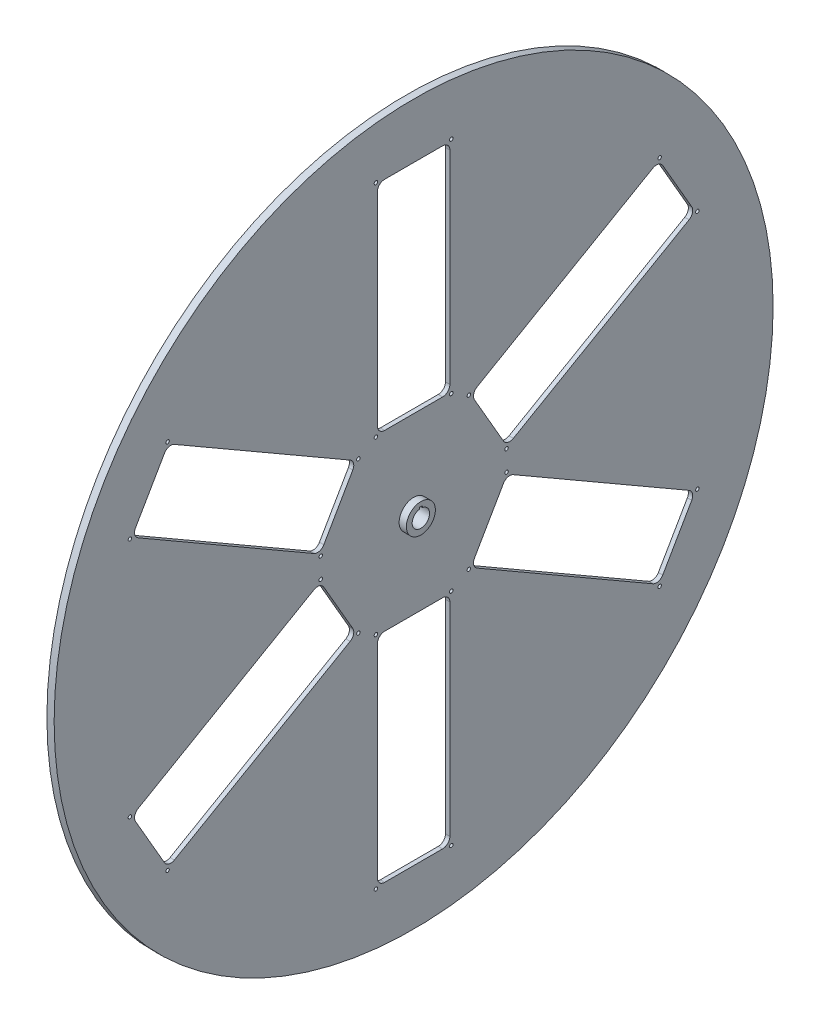
SolidWorks part; units mm, degrees
material "AISI 304"
ref_plane "Front Plane" through (0, 0, 0) normal (0, 0, 1) x (1, 0, 0)
ref_plane "Top Plane" through (0, 0, 0) normal (0, 1, 0) x (1, 0, 0)
ref_plane "Right Plane" through (0, 0, 0) normal (1, 0, 0) x (0, 0, -1)
sketch "Sketch1" plane through (0, 0, 0) normal (1, 0, 0) x (0, 0, -1)
  circle A0 centre (0, 0) radius 250
  dimension "D1" = 500
extrude "Boss-Extrude1" add sketch "Sketch1" along normal blind 5
sketch "Sketch5" plane through (0, 0, 0) normal (-1, 0, 0) x (0, 0, 1)
  line L0 (0, 0) -> (0, 425.8761) construction
  line L2 (-25, 210) -> (25, 210)
  line L3 (-25, 210) -> (-25, 60)
  line L4 (-25, 60) -> (25, 60)
  line L5 (25, 210) -> (25, 60)
  line L6 (-25, 210) -> (25, 60) construction
  line L7 (-25, 60) -> (25, 210) construction
  point P3 (0, 135)
  dimension "D1" = 50
  dimension "D2" = 60
  dimension "D3" = 150
extrude "Cut-Extrude1" cut sketch "Sketch5" against normal through all
pattern_circular "CirPattern1" count 6 over 360 about axis through (0, 0, 0) along (1, 0, 0) of "Cut-Extrude1"
sketch "Sketch6" plane through (0, 0, 0) normal (-1, 0, 0) x (0, 0, 1)
  line L8 (-30, 55) -> (30, 55)
  line L9 (30, 55) -> (30, 215)
  line L10 (-30, 215) -> (-30, 55)
  line L11 (30, 215) -> (-30, 215)
  line L12 (-30, 55) -> (30, 55)
  line L13 (30, 55) -> (30, 215)
  line L14 (-30, 215) -> (-30, 55)
  line L15 (30, 215) -> (-30, 215)
  dimension "D1" = 5
extrude "Cut-Extrude2" cut sketch "Sketch6" against normal blind 2
sketch "Sketch7" plane through (2, 0, 0) normal (-1, 0, 0) x (0, 0, 1)
  circle A0 centre (-26, 211) radius 1
  circle A1 centre (26, 211) radius 1
  circle A2 centre (-26, 59) radius 1
  circle A3 centre (26, 59) radius 1
extrude "Cut-Extrude3" cut sketch "Sketch7" against normal blind 10
hole_wizard "M2 Clearance Hole1" positions "Sketch8" profile "Sketch9" hole size "M2" standard "GB"
sketch "Sketch8" plane through (2, 0, 0) normal (-1, 0, 0) x (0, 0, 1)
  point P0 (-26, 59)
  point P3 (-26, 211)
  point P6 (26, 211)
  point P9 (26, 59)
sketch "Sketch9" plane through (2, 59, -26) normal (0, 1, 0) x (0, 0, 1)
  line L0 (0, 0) -> (0, 8.221)
  line L1 (0, 8.221) -> (1.2, 7.5)
  line L2 (1.2, 7.5) -> (1.2, 0)
  line L5 (1.2, 0) -> (0, 0)
  line L10 (0, 8.221) -> (-1.2, 7.5) construction
  line L11 (0, -6.35) -> (0, 107.95) construction
  dimension "孔直径" = 2.4
  dimension "孔深度" = 7.5
  dimension "导头角度" = 118
pattern_circular "CirPattern2" count 6 over 360 about axis through (0, 0, 0) along (1, 0, 0) of "Cut-Extrude2", "Cut-Extrude3", "M2 Clearance Hole1"
fillet "Fillet1" radius 5 24 edges at (1, 55, 30) (1, 215, 30) (1, 215, -30) (1, 55, -30) (1, 53.4808, -32.6314) (1, 133.4808, -171.1955) (1, 81.5192, -201.1955) (1, 1.5192, -62.6314) (1, 1.5192, 62.6314) (1, 81.5192, 201.1955) (1, 133.4808, 171.1955) (1, 53.4808, 32.6314) (1, -53.4808, 32.6314) (1, -133.4808, 171.1955) (1, -81.5192, 201.1955) (1, -1.5192, 62.6314) (1, -55, -30) (1, -215, -30) (1, -215, 30) (1, -55, 30) (1, -1.5192, -62.6314) (1, -133.4808, -171.1955) (1, -53.4808, -32.6314) (1, -81.5192, -201.1955)
fillet "Fillet2" radius 5 24 edges at (3.5, 60, 25) (3.5, 60, -25) (3.5, 210, -25) (3.5, 210, 25) (3.5, 51.6506, -39.4615) (3.5, 8.3494, -64.4615) (3.5, 126.6506, -169.3653) (3.5, 8.3494, 64.4615) (3.5, 51.6506, 39.4615) (3.5, 126.6506, 169.3653) (3.5, 83.3494, 194.3653) (3.5, -51.6506, 39.4615) (3.5, -8.3494, 64.4615) (3.5, -83.3494, 194.3653) (3.5, -126.6506, 169.3653) (3.5, -60, -25) (3.5, -60, 25) (3.5, -210, 25) (3.5, -210, -25) (3.5, 83.3494, -194.3653) (3.5, -8.3494, -64.4615) (3.5, -51.6506, -39.4615) (3.5, -126.6506, -169.3653) (3.5, -83.3494, -194.3653)
sketch "Sketch11" plane through (0, 0, 0) normal (-1, 0, 0) x (0, 0, 1)
  circle A0 centre (0, 0) radius 6
  dimension "D1" = 12
extrude "Cut-Extrude4" cut sketch "Sketch11" against normal through all
sketch "Sketch12" plane through (0, 0, 0) normal (-1, 0, 0) x (0, 0, 1)
  circle A0 centre (0, 0) radius 6
  circle A1 centre (0, 0) radius 10
  dimension "D1" = 20
extrude "Boss-Extrude2" add sketch "Sketch12" against normal blind 15 from offset 5
sketch "Sketch13" plane through (-5, 0, 0) normal (-1, 0, 0) x (0, 0, 1)
  line L0 (0, 0) -> (0, 13.5117) construction
  line L2 (-1, 7) -> (1, 7)
  line L3 (-1, 7) -> (-1, 5)
  line L4 (-1, 5) -> (1, 5)
  line L5 (1, 7) -> (1, 5)
  line L6 (-1, 7) -> (1, 5) construction
  line L7 (-1, 5) -> (1, 7) construction
  circle A0 centre (0, 0) radius 6 construction
  point P3 (0, 6)
  dimension "D1" = 2
  dimension "D2" = 2
extrude "Cut-Extrude5" cut sketch "Sketch13" against normal through all
sketch "Sketch14" plane through (0, 0, 0) normal (-1, 0, 0) x (0, 0, 1)
  circle A0 centre (0, 0) radius 250 construction
  circle A1 centre (0, 0) radius 250
  circle A2 centre (0, 0) radius 248
  dimension "D1" = 2
extrude "Cut-Extrude6" cut sketch "Sketch14" against normal through all
